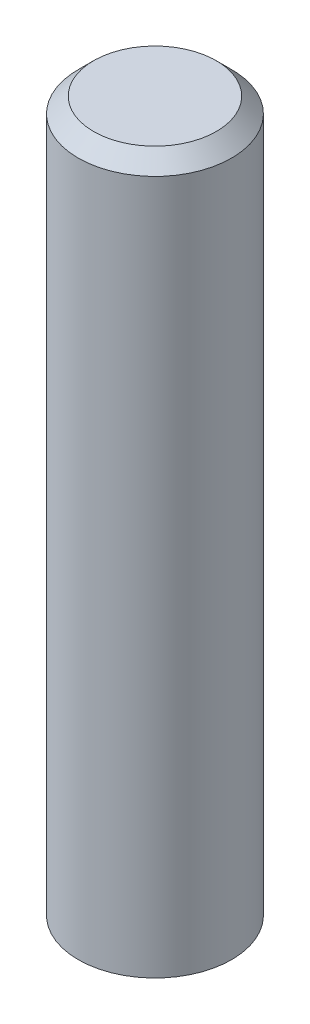
SolidWorks part; units mm, degrees
ref_plane "Front Plane" through (0, 0, 0) normal (0, 0, 1) x (1, 0, 0)
ref_plane "Top Plane" through (0, 0, 0) normal (0, 1, 0) x (1, 0, 0)
ref_plane "Right Plane" through (0, 0, 0) normal (1, 0, 0) x (0, 0, -1)
sketch "Sketch 1" plane through (0, 0, 0) normal (0, 1, 0) x (1, 0, 0)
  circle A0 centre (0, 0) radius 10
  dimension "D1" = 20
extrude "Boss-Extrude 1" add sketch "Sketch 1" along normal blind 92.5
ref_plane "Plane 1" through (0, 0, -6.5) normal (0, 0, 1) x (1, 0, 0)
sketch "Sketch 2" plane through (0, 0, -6.5) normal (0, 0, 1) x (1, 0, 0)
  line L0 (0, 63.5) -> (0, 85.5) construction
  line L1 (-3, 63.5) -> (-3, 85.5)
  line L2 (3, 63.5) -> (3, 85.5)
  line L3 (10, 92.5) -> (-10, 92.5) construction
  arc A0 (-3, 63.5) -> (3, 63.5) centre (0, 63.5) ccw
  arc A1 (3, 85.5) -> (-3, 85.5) centre (0, 85.5) ccw
  point P3 (0, 74.5)
  point P8 (0, 88.5)
  point P9 (0, 60.5)
  dimension "D1" = 28
  dimension "D2" = 6
  dimension "D3" = 4
extrude "Cut-Extrude 1" cut sketch "Sketch 2" against normal through all
chamfer "Chamfer 1" distance 2 angle 45 1 edges at (0, 92.5, 10)
